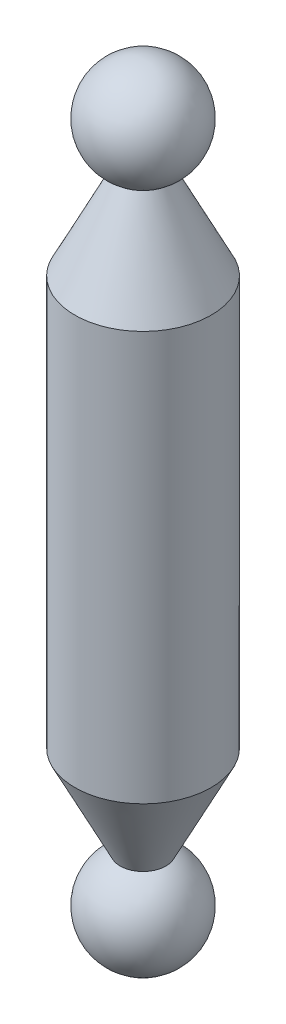
SolidWorks part; units mm, degrees
ref_plane "Front Plane" through (0, 0, 0) normal (0, 0, 1) x (1, 0, 0)
ref_plane "Top Plane" through (0, 0, 0) normal (0, 1, 0) x (1, 0, 0)
ref_plane "Right Plane" through (0, 0, 0) normal (1, 0, 0) x (0, 0, -1)
sketch "Sketch1" plane through (0, 0, 0) normal (0, 0, 1) x (1, 0, 0)
  line L0 (0, -7.5) -> (0, 107.5) construction
  line L1 (-3.3541, 93.2918) -> (-10, 80)
  line L2 (-10, 80) -> (-10, 20)
  line L3 (-10, 20) -> (-3.3541, 6.7082)
  line L4 (0, 107.5) -> (0, -7.5)
  arc A0 (-3.3541, 6.7082) -> (0, -7.5) centre (0, 0) ccw
  arc A1 (0, 107.5) -> (-3.3541, 93.2918) centre (0, 100) ccw
  dimension "D1" = 100
  dimension "D2" = 15
  dimension "D3" = 15
  dimension "D4" = 20
  dimension "D5" = 20
  dimension "D6" = 20
revolve "Revolve1" add sketch "Sketch1" angle 360 about L0
